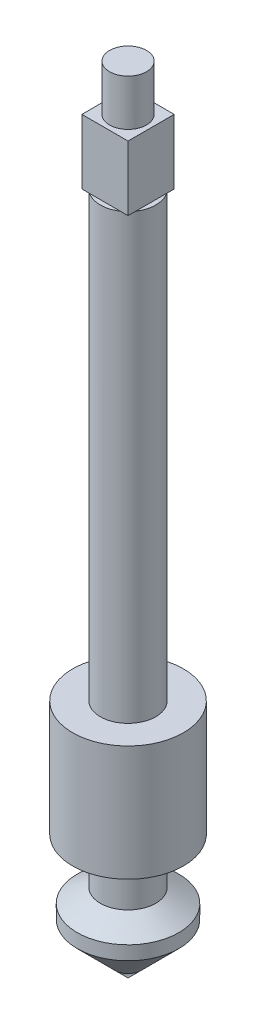
SolidWorks part; units mm, degrees
ref_plane "Front Plane" through (0, 0, 0) normal (0, 0, 1) x (1, 0, 0)
ref_plane "Top Plane" through (0, 0, 0) normal (0, 1, 0) x (1, 0, 0)
ref_plane "Right Plane" through (0, 0, 0) normal (1, 0, 0) x (0, 0, -1)
sketch "Sketch1" plane through (0, 0, 0) normal (0, 0, 1) x (1, 0, 0)
  line L0 (0, -1000) -> (0, 49000) construction
  line L1 (0, 0) -> (-11, 11)
  line L2 (-11, 11) -> (-11, 14)
  line L3 (-11, 14) -> (-6, 17)
  line L4 (-6, 17) -> (-6, 27)
  line L5 (-6, 27) -> (-12, 27)
  line L6 (-12, 27) -> (-12, 52)
  line L7 (-12, 52) -> (-6, 52)
  line L8 (-6, 52) -> (-6, 148)
  line L9 (-6, 148) -> (0, 148)
  line L10 (0, 0) -> (0, 148)
  dimension "D1" = 45
  dimension "D2" = 11
  dimension "D3" = 3
  dimension "D4" = 3
  dimension "D5" = 6
  dimension "D6" = 12
  dimension "D7" = 25
  dimension "D8" = 13
  dimension "D9" = 96
revolve "Revolve1" add sketch "Sketch1" angle 360 about L0
sketch "Sketch2" plane through (0, 148, 0) normal (0, 1, 0) x (1, 0, 0)
  line L1 (-5, -5) -> (5, -5)
  line L2 (-5, -5) -> (-5, 5)
  line L3 (-5, 5) -> (5, 5)
  line L4 (5, -5) -> (5, 5)
  line L5 (-5, -5) -> (5, 5) construction
  line L6 (-5, 5) -> (5, -5) construction
  point P0 (0, 0)
  dimension "D1" = 10
extrude "Boss-Extrude1" add sketch "Sketch2" along normal blind 14
sketch "Sketch3" plane through (0, 162, 0) normal (0, 1, 0) x (1, 0, 0)
  circle A0 centre (0, 0) radius 4
  dimension "D1" = 8
extrude "Boss-Extrude2" add sketch "Sketch3" along normal blind 10
